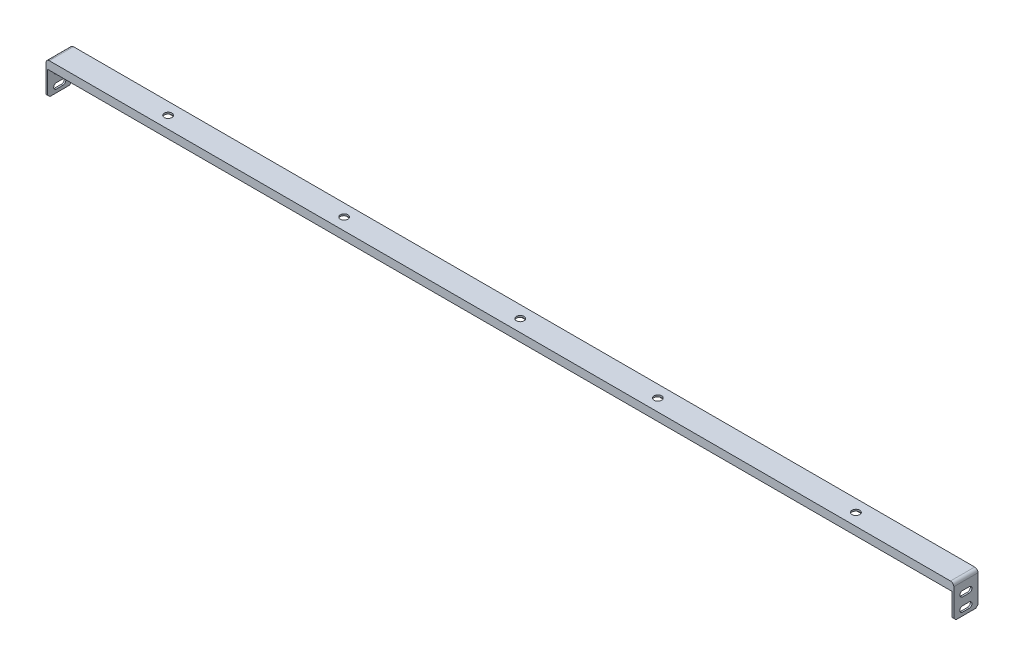
from build123d import *

# Parameters (mm, degrees)
EXTRUDE_1_DEPTH       = 22
SKETCH_2_W            = 822
SKETCH_2_H            = 6
EXTRUDE_2_DEPTH       = 2
SKETCH_3_W            = 822
SKETCH_3_H            = 6
EXTRUDE_3_DEPTH       = 2
CUT_EXTRUDE_1_DEPTH   = 826.838361909
CHAMFER_1_SIZE        = 2
FILLET_1_R            = 3
HOLE_WIZARD_7_0_7_1_D = 7


with BuildPart() as part:
    # 草图1 → 凸台-拉伸1 (new body)
    with BuildSketch(Plane.XY):
        Polygon((0, 0), (0, 30), (825, 30), (825, 0), (823.5, 0), (823.5, 28.5), (1.5, 28.5), (1.5, 0), align=None)
    extrude(amount=EXTRUDE_1_DEPTH)

    # 草图2 → 凸台-拉伸2 (add)
    with BuildSketch(Plane.XY.offset(22)):
        with Locations((412.5, 25.5)):
            Rectangle(SKETCH_2_W, SKETCH_2_H)
    extrude(amount=-EXTRUDE_2_DEPTH)

    # 草图3 → 凸台-拉伸3 (add)
    with BuildSketch(Plane(origin=(0, 0, 0), x_dir=(-1, 0, 0), z_dir=(0, 0, -1))):
        with Locations((-412.5, 25.5)):
            Rectangle(SKETCH_3_W, SKETCH_3_H)
    extrude(amount=-EXTRUDE_3_DEPTH)

    # 草图5 → 切除-拉伸1 (cut, through all)
    with BuildSketch(Plane.ZY):
        with BuildLine():
            Line((8, 20), (14, 20))
            ThreePointArc((14, 20), (16.5, 17.5), (14, 15))
            Line((14, 15), (8, 15))
            ThreePointArc((8, 15), (5.5, 17.5), (8, 20))
        make_face()
        with BuildLine():
            Line((8, 8), (14, 8))
            ThreePointArc((14, 8), (16.5, 5.5), (14, 3))
            Line((14, 3), (8, 3))
            ThreePointArc((8, 3), (5.5, 5.5), (8, 8))
        make_face()
    extrude(amount=-CUT_EXTRUDE_1_DEPTH, mode=Mode.SUBTRACT)

    # 倒角1
    chamfer_1_edges = [part.edges().sort_by_distance(p)[0] for p in [
        (0.75, 0, 0),
        (824.25, 0, 22),
        (0.75, 0, 22),
        (824.25, 0, 0),
    ]]
    chamfer(chamfer_1_edges, length=CHAMFER_1_SIZE)

    # 圆角1
    fillet_1_edges = [part.edges().sort_by_distance(p)[0] for p in [
        (0, 30, 11),
        (825, 30, 11),
    ]]
    fillet(fillet_1_edges, radius=FILLET_1_R)

    # Ø7.0 (7) 直径孔1 (through all)
    with Locations(Plane(origin=(0, 28.5, 0), x_dir=(-1, 0, 0), z_dir=(0, -1, 0))):
        with Locations((-100, -11), (-260, -11), (-420, -11), (-545, -11), (-725, -11)):
            Hole(HOLE_WIZARD_7_0_7_1_D / 2)


solid = part.part
